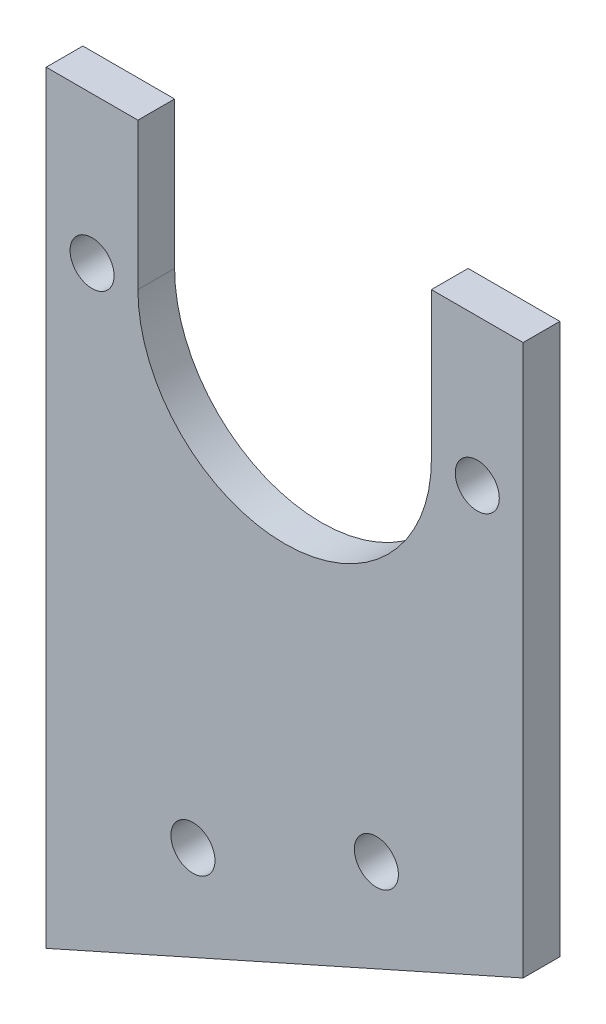
SolidWorks part; units mm, degrees
ref_plane "前视基准面" through (0, 0, 0) normal (0, 0, 1) x (1, 0, 0)
ref_plane "上视基准面" through (0, 0, 0) normal (0, 1, 0) x (1, 0, 0)
ref_plane "右视基准面" through (0, 0, 0) normal (1, 0, 0) x (0, 0, -1)
sketch "草图1" plane through (0, 0, 0) normal (0, 0, 1) x (1, 0, 0)
  line L0 (130, 208) -> (130, 58)
  line L1 (0, 208) -> (25, 208)
  line L2 (0, 0) -> (0, 208)
  line L3 (130, 58) -> (0, 0)
  line L4 (105, 168) -> (105, 208)
  line L5 (25, 168) -> (25, 208)
  line L6 (105, 208) -> (130, 208)
  arc A0 (25, 168) -> (105, 168) centre (65, 168) ccw
  circle A1 centre (117.5, 168) radius 6
  circle A2 centre (12.5, 168) radius 6
  circle A3 centre (40, 43.72) radius 6
  circle A4 centre (90, 65.43) radius 6
  dimension "D1" = 40
  dimension "D2" = 52.5
  dimension "D3" = 52.5
extrude "凸台-拉伸1" add sketch "草图1" along normal blind 10
